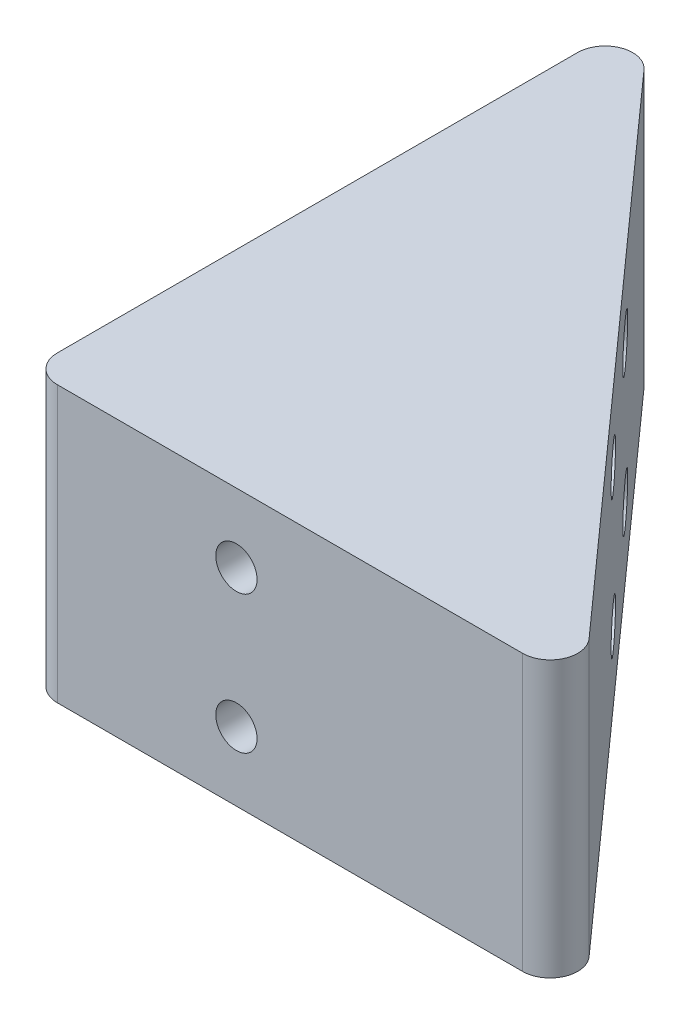
from build123d import *

# Parameters (mm, degrees)
EXTRUDE_1_DEPTH     = 20
FILLET_1_R          = 2
SKETCH_2_R          = 1.5
CUT_EXTRUDE_1_DEPTH = 60.760642304
SKETCH_3_R          = 1.5
CUT_EXTRUDE_2_DEPTH = 60.760642304


with BuildPart() as part:
    # 草图1 → 凸台-拉伸1 (new body)
    with BuildSketch(Plane(origin=(0, 0, 0), x_dir=(1, 0, 0), z_dir=(0, 1, 0))):
        Polygon((0, 45), (0, 0), (40.249223595, 0), align=None)
    extrude(amount=EXTRUDE_1_DEPTH)

    # 圆角1
    fillet_1_edges = [part.edges().sort_by_distance(p)[0] for p in [
        (40.249223595, 10, 0),
        (0, 10, 0),
        (0, 10, -45),
    ]]
    fillet(fillet_1_edges, radius=FILLET_1_R)

    # 草图2 → 切除-拉伸1 (cut, through all)
    with BuildSketch(Plane.ZY):
        with Locations((-20, 15)):
            Circle(SKETCH_2_R)
        with Locations((-20, 5)):
            Circle(SKETCH_2_R)
    extrude(amount=-CUT_EXTRUDE_1_DEPTH, mode=Mode.SUBTRACT)

    # 草图3 → 切除-拉伸2 (cut, through all)
    with BuildSketch(Plane.XY):
        with Locations((15, 15)):
            Circle(SKETCH_3_R)
        with Locations((15, 5)):
            Circle(SKETCH_3_R)
    extrude(amount=-CUT_EXTRUDE_2_DEPTH, mode=Mode.SUBTRACT)


solid = part.part
